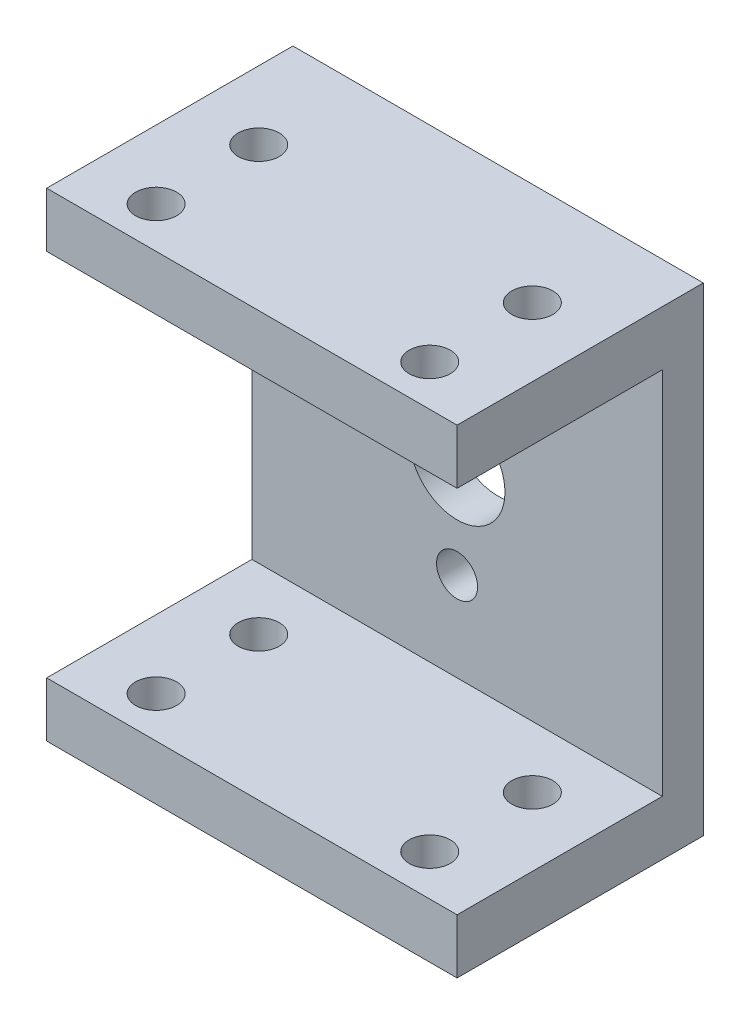
SolidWorks part; units mm, degrees
ref_plane "Front Plane" through (0, 0, 0) normal (0, 0, 1) x (1, 0, 0)
ref_plane "Top Plane" through (0, 0, 0) normal (0, 1, 0) x (1, 0, 0)
ref_plane "Right Plane" through (0, 0, 0) normal (1, 0, 0) x (0, 0, -1)
other "Configuration Table"
sketch "Sketch1" plane through (0, 0, 0) normal (0, 0, 1) x (1, 0, 0)
  line L1 (-15, -17.5) -> (15, -17.5)
  line L2 (-15, -17.5) -> (-15, 17.5)
  line L3 (-15, 17.5) -> (15, 17.5)
  line L4 (15, -17.5) -> (15, 17.5)
  line L5 (0, 17.5) -> (0, -17.5) construction
  line L6 (-15, 0) -> (15, 0) construction
  circle A1 centre (0, 0) radius 3.5
  circle A2 centre (0, 0) radius 7 construction
  circle A3 centre (0, 7) radius 1.5
  circle A4 centre (0, -7) radius 1.5
  point P0 (0, 0)
  dimension "D1" = 7
  dimension "D2" = 14
  dimension "D3" = 3
  dimension "D4" = 35
  dimension "D5" = 30
extrude "Boss-Extrude1" add sketch "Sketch1" along normal blind 3
sketch "Sketch2" plane through (0, 0, 3) normal (0, 0, 1) x (1, 0, 0)
  line L0 (15, -17.5) -> (15, 17.5) construction
  line L1 (-15, 17.5) -> (15, 17.5)
  line L2 (-15, 17.5) -> (-15, 13.5)
  line L3 (-15, 13.5) -> (15, 13.5)
  line L4 (15, 17.5) -> (15, 13.5)
  line L6 (0, 0) -> (26.0855, 0) construction
  line L7 (15, -17.5) -> (15, -13.5)
  line L8 (-15, -13.5) -> (15, -13.5)
  line L9 (-15, -17.5) -> (-15, -13.5)
  line L10 (-15, -17.5) -> (15, -17.5)
  dimension "D1" = 4
extrude "Boss-Extrude2" add sketch "Sketch2" along normal blind 15
sketch "Sketch4" plane through (0, 13.5, 0) normal (0, -1, 0) x (1, 0, 0)
  line L0 (-15, 18) -> (15, 18) construction
  line L1 (-10, 7.5) -> (10, 7.5) construction
  line L2 (-10, 7.5) -> (-10, 15) construction
  line L3 (-10, 15) -> (10, 15) construction
  line L4 (10, 7.5) -> (10, 15) construction
  line L5 (0, 15) -> (0, 7.5) construction
  line L6 (-10, 11.25) -> (10, 11.25) construction
  circle A0 centre (-10, 15) radius 1.5
  circle A1 centre (10, 15) radius 1.5
  circle A2 centre (10, 7.5) radius 1.5
  circle A3 centre (-10, 7.5) radius 1.5
  point P0 (0, 11.25)
  dimension "D4" = 3
  dimension "D1" = 20
  dimension "D2" = 7.5
  dimension "D3" = 3
extrude "Cut-Extrude1" cut sketch "Sketch4" against normal blind 15
mirror "Mirror1" about plane through (0, 0, 0) normal (0, 1, 0) of "Cut-Extrude1"
